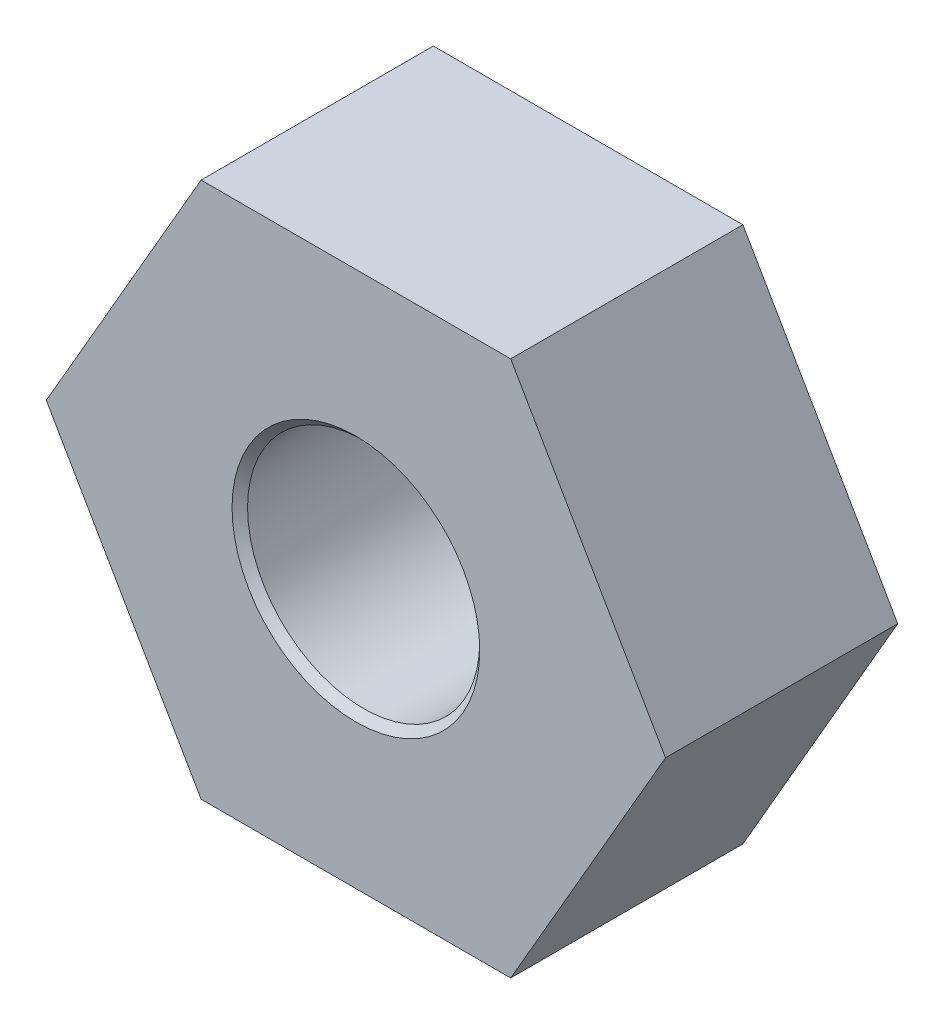
from build123d import *

# Parameters (mm, degrees)
SKETCH1_R           = 1.5
BOSS_EXTRUDE1_DEPTH = 3
CHAMFER1_SIZE       = 0.1


with BuildPart() as part:
    # Sketch1 → Boss-Extrude1 (new body)
    with BuildSketch(Plane.XY):
        Polygon((2, -3.464101615), (4, 0), (2, 3.464101615), (-2, 3.464101615), (-4, 0), (-2, -3.464101615), align=None)
        Circle(SKETCH1_R, mode=Mode.SUBTRACT)
    extrude(amount=BOSS_EXTRUDE1_DEPTH)

    # Chamfer1
    chamfer1_edges = [part.edges().sort_by_distance(p)[0] for p in [
        (-1.5, 0, 0),
        (-1.5, 0, 3),
    ]]
    chamfer(chamfer1_edges, length=CHAMFER1_SIZE)


solid = part.part
